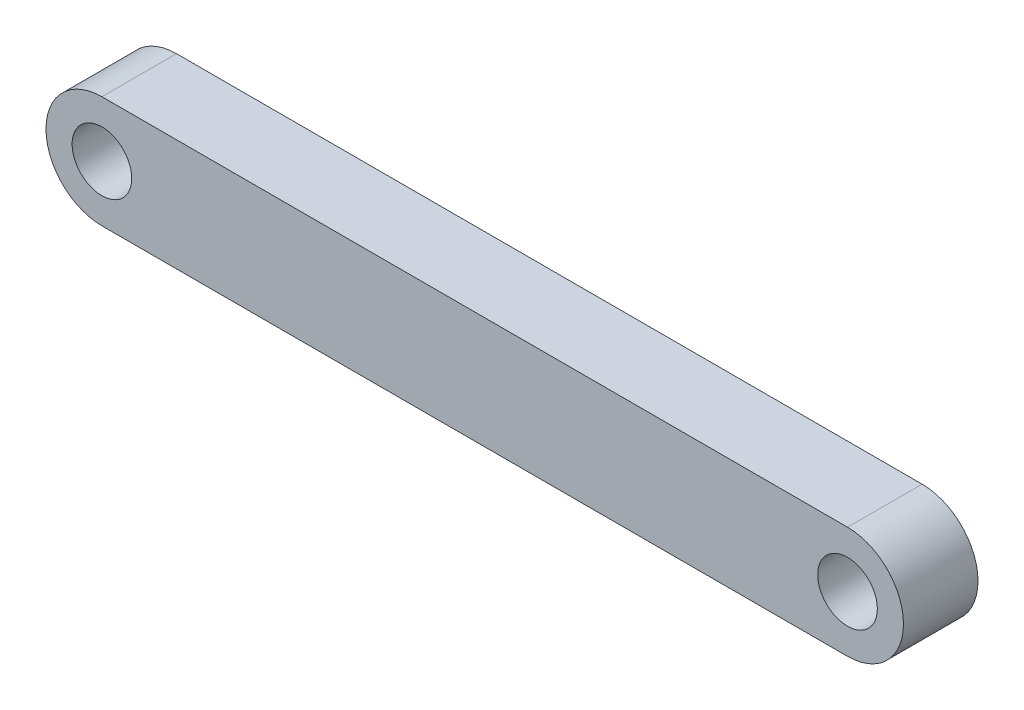
from build123d import *

# Parameters (mm, degrees)
SKETCH1_R           = 4
BOSS_EXTRUDE1_DEPTH = 10


with BuildPart() as part:
    # Sketch1 → Boss-Extrude1 (new body)
    with BuildSketch(Plane.XY):
        with BuildLine():
            Line((0, 7.5), (100, 7.5))
            ThreePointArc((100, 7.5), (107.5, 0), (100, -7.5))
            Line((100, -7.5), (0, -7.5))
            ThreePointArc((0, -7.5), (-7.5, 0), (0, 7.5))
        make_face()
        Circle(SKETCH1_R, mode=Mode.SUBTRACT)
        with Locations((100, 0)):
            Circle(SKETCH1_R, mode=Mode.SUBTRACT)
    extrude(amount=BOSS_EXTRUDE1_DEPTH)


solid = part.part
